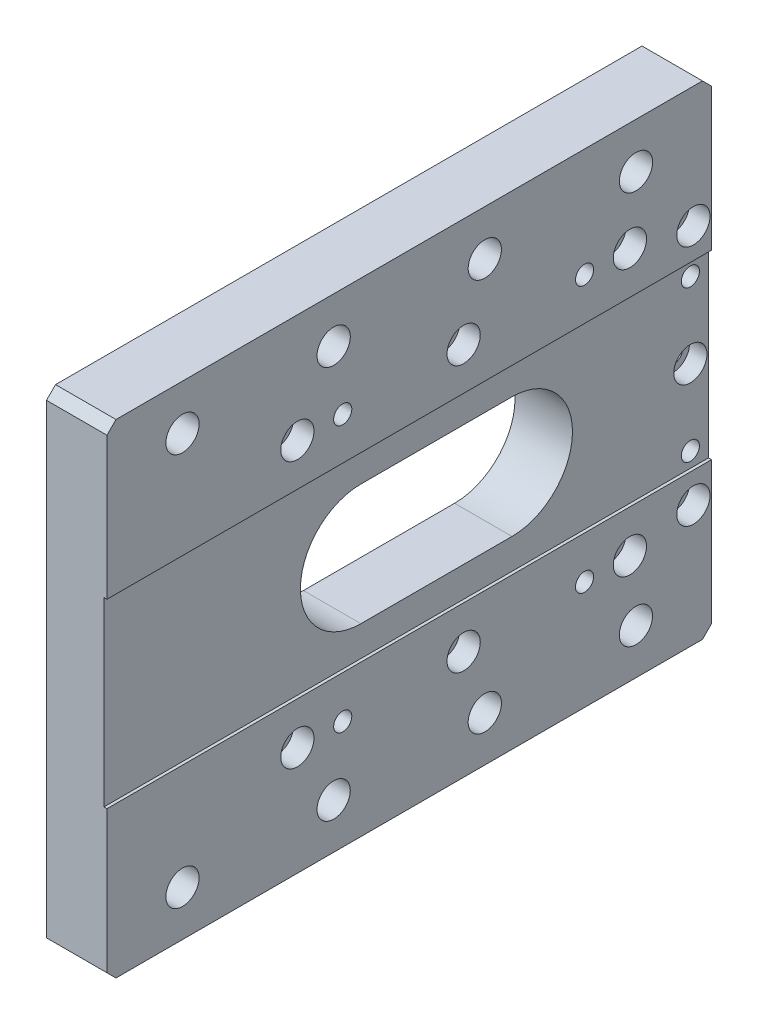
from build123d import *

# Parameters (mm, degrees)
SKETCH4_W                                        = 200
SKETCH4_H                                        = 160
SKETCH4_R                                        = 5.5
BOSS_EXTRUDE4_DEPTH                              = 20
HOLE_SIZE_PER_HEX_SOCKET_SCREW_TYPE1_D           = 6.6
HOLE_SIZE_PER_HEX_SOCKET_SCREW_TYPE1_CBORE_D     = 11
HOLE_SIZE_PER_HEX_SOCKET_SCREW_TYPE1_CBORE_DEPTH = 6.8
F_6_0_6_DIAMETER_HOLE1_D                         = 6
SKETCH10_W                                       = 200
SKETCH10_H                                       = 60
CUT_EXTRUDE4_DEPTH                               = 1
CHAMFER1_SIZE                                    = 3


with BuildPart() as part:
    # Sketch4 → Boss-Extrude4 (new body)
    with BuildSketch(Plane(origin=(0, 0, 0), x_dir=(0, 0, -1), z_dir=(1, 0, 0))):
        with Locations((-100, 0)):
            Rectangle(SKETCH4_W, SKETCH4_H)
        with Locations((-125, -65)):
            Circle(SKETCH4_R, mode=Mode.SUBTRACT)
        with Locations((-75, -65)):
            Circle(SKETCH4_R, mode=Mode.SUBTRACT)
        with Locations((-25, -65)):
            Circle(SKETCH4_R, mode=Mode.SUBTRACT)
        with Locations(Location((-125, 65, 0), (0, 0, 180))):
            Circle(SKETCH4_R, mode=Mode.SUBTRACT)
        with Locations(Location((-75, 65, 0), (0, 0, 180))):
            Circle(SKETCH4_R, mode=Mode.SUBTRACT)
        with Locations(Location((-25, 65, 0), (0, 0, 180))):
            Circle(SKETCH4_R, mode=Mode.SUBTRACT)
        with Locations((-175, -65)):
            Circle(SKETCH4_R, mode=Mode.SUBTRACT)
        with Locations((-175, 65)):
            Circle(SKETCH4_R, mode=Mode.SUBTRACT)
        with BuildLine():
            Line((-65, -20), (-115, -20))
            ThreePointArc((-115, -20), (-135, 0), (-115, 20))
            Line((-115, 20), (-65, 20))
            ThreePointArc((-65, 20), (-45, 0), (-65, -20))
        make_face(mode=Mode.SUBTRACT)
    extrude(amount=BOSS_EXTRUDE4_DEPTH)

    # Hole size per hex socket screw type1 (through all)
    with Locations(Plane(origin=(20, 0, 0), x_dir=(0, 0, -1), z_dir=(1, 0, 0))):
        with Locations((-6, 40), (-6, 0), (-6, -40), (-27, -44), (-82, -44), (-137, -44), (-27, 44), (-82, 44), (-137, 44)):
            CounterBoreHole(HOLE_SIZE_PER_HEX_SOCKET_SCREW_TYPE1_D / 2, HOLE_SIZE_PER_HEX_SOCKET_SCREW_TYPE1_CBORE_D / 2, HOLE_SIZE_PER_HEX_SOCKET_SCREW_TYPE1_CBORE_DEPTH)

    # Ø6.0 (6) Diameter Hole1 (through all)
    with Locations(Plane(origin=(20, 0, 0), x_dir=(0, 0, -1), z_dir=(1, 0, 0))):
        with Locations((-6, 25), (-6, -25), (-42, -44), (-122, -44), (-122, 44), (-42, 44)):
            Hole(F_6_0_6_DIAMETER_HOLE1_D / 2)

    # Sketch10 → Cut-Extrude4 (cut)
    with BuildSketch(Plane(origin=(20, 0, 0), x_dir=(0, 0, -1), z_dir=(1, 0, 0))):
        with Locations((-100, 0)):
            Rectangle(SKETCH10_W, SKETCH10_H)
    extrude(amount=-CUT_EXTRUDE4_DEPTH, mode=Mode.SUBTRACT)

    # Chamfer1
    chamfer1_edges = [part.edges().sort_by_distance(p)[0] for p in [
        (10, 80, 200),
        (10, 80, 0),
        (10, -80, 0),
        (10, -80, 200),
    ]]
    chamfer(chamfer1_edges, length=CHAMFER1_SIZE)


solid = part.part
